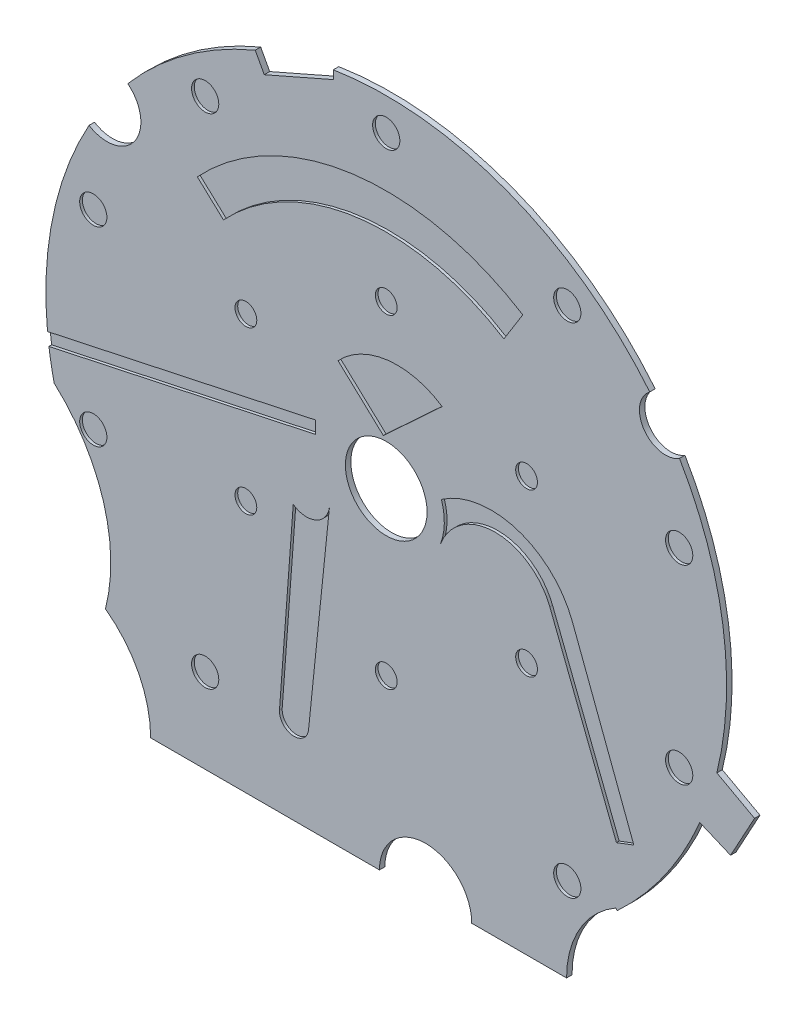
from build123d import *

# Parameters (mm, degrees)
BOSS_EXTRUDE2_DEPTH = 0.2
SKETCH4_R           = 1.5
CUT_EXTRUDE1_DEPTH  = 0.2
SKETCH5_R           = 0.5
CUT_EXTRUDE2_DEPTH  = 0.1
SKETCH6_R           = 0.4
CUT_EXTRUDE3_DEPTH  = 0.1
CUT_EXTRUDE6_DEPTH  = 0.1


with BuildPart() as part:
    # Sketch3 → Boss-Extrude2 (new body)
    with BuildSketch(Plane.XY):
        with BuildLine():
            Line((-8.650876673, -12.25407413), (-0.248745803, -12.25407413))
            ThreePointArc((-0.248745803, -12.25407413), (1.445834978, -10.55949335), (3.140415758, -12.25407413))
            Line((3.140415758, -12.25407413), (6.622856994, -12.25407413))
            ThreePointArc((6.622856994, -12.25407413), (7.105995692, -10.448666248), (8.426264063, -9.125861633))
            Line((8.426264063, -9.125861633), (8.479800816, -9.183843319))
            ThreePointArc((8.479800816, -9.183843319), (10.228299659, -7.185533111), (11.515265421, -4.862989028))
            Line((11.515265421, -4.862989028), (12.645034643, -5.340099639))
            Line((12.645034643, -5.340099639), (13.525538654, -3.725359149))
            Line((13.525538654, -3.725359149), (12.14183381, -2.970836876))
            ThreePointArc((12.14183381, -2.970836876), (12.366623578, 1.821159325), (10.769957457, 6.344920517))
            ThreePointArc((10.769957457, 6.344920517), (9.469693231, 6.602612743), (9.677487695, 7.91177805))
            ThreePointArc((9.677487695, 7.91177805), (4.458067099, 11.67799802), (-1.943326583, 12.348015298))
            Line((-1.943326583, 12.348015298), (-1.943326583, 12.035386554))
            Line((-1.943326583, 12.035386554), (-4.479228025, 10.922703455))
            Line((-4.479228025, 10.922703455), (-4.810432032, 11.537319605))
            ThreePointArc((-4.810432032, 11.537319605), (-7.351587465, 10.109607398), (-9.493012594, 8.132202155))
            ThreePointArc((-9.493012594, 8.132202155), (-9.234137218, 6.438374568), (-10.912999752, 6.095607961))
            ThreePointArc((-10.912999752, 6.095607961), (-12.370451822, 1.794971228), (-12.195428383, -2.742540164))
            ThreePointArc((-12.195428383, -2.742540164), (-10.385309853, -5.600254803), (-10.310731268, -8.98219213))
            ThreePointArc((-10.310731268, -8.98219213), (-9.089572731, -10.419658072), (-8.650876673, -12.25407413))
        make_face()
    extrude(amount=BOSS_EXTRUDE2_DEPTH)

    # Sketch4 → Cut-Extrude1 (cut)
    with BuildSketch(Plane.XY.offset(0.2)):
        Circle(SKETCH4_R)
    extrude(amount=-CUT_EXTRUDE1_DEPTH, mode=Mode.SUBTRACT)

    # Sketch5 → Cut-Extrude2 (cut)
    with BuildSketch(Plane.XY.offset(0.2)):
        with Locations((0, 11.311857504)):
            Circle(SKETCH5_R)
        with Locations((6.648943017, 9.151484959)):
            Circle(SKETCH5_R)
        with Locations((10.75821579, 3.495556207)):
            Circle(SKETCH5_R)
        with Locations((10.75821579, -3.495556207)):
            Circle(SKETCH5_R)
        with Locations((6.648943017, -9.151484959)):
            Circle(SKETCH5_R)
        with Locations((-6.648943017, -9.151484959)):
            Circle(SKETCH5_R)
        with Locations((-10.75821579, -3.495556207)):
            Circle(SKETCH5_R)
        with Locations((-10.75821579, 3.495556207)):
            Circle(SKETCH5_R)
        with Locations((-6.648943017, 9.151484959)):
            Circle(SKETCH5_R)
    extrude(amount=-CUT_EXTRUDE2_DEPTH, mode=Mode.SUBTRACT)

    # Sketch6 → Cut-Extrude3 (cut)
    with BuildSketch(Plane.XY.offset(0.2)):
        with Locations((0, 5.951320454)):
            Circle(SKETCH6_R)
        with Locations((5.153994699, 2.975660227)):
            Circle(SKETCH6_R)
        with Locations((5.153994699, -2.975660227)):
            Circle(SKETCH6_R)
        with Locations((0, -5.951320454)):
            Circle(SKETCH6_R)
        with Locations((-5.153994699, -2.975660227)):
            Circle(SKETCH6_R)
        with Locations((-5.153994699, 2.975660227)):
            Circle(SKETCH6_R)
    extrude(amount=-CUT_EXTRUDE3_DEPTH, mode=Mode.SUBTRACT)

    # Sketch7 → Cut-Extrude6 (cut)
    with BuildSketch(Plane.XY.offset(0.2)):
        with BuildLine():
            Line((-6.937396584, 6.446885446), (-6.51899849, 6.058070341))
            ThreePointArc((-6.51899849, 6.058070341), (-1.17077586, 8.821952247), (4.713219322, 7.548716526))
            Line((4.713219322, 7.548716526), (5.01572008, 8.033203309))
            ThreePointArc((5.01572008, 8.033203309), (-1.245917829, 9.388157012), (-6.937396584, 6.446885446))
        make_face()
        with BuildLine():
            Line((-6.51899849, 6.058070341), (-5.97717014, 5.554552161))
            ThreePointArc((-5.97717014, 5.554552161), (-1.073466502, 8.088713263), (4.321478804, 6.921302879))
            Line((4.321478804, 6.921302879), (4.713219322, 7.548716526))
            ThreePointArc((4.713219322, 7.548716526), (-1.17077586, 8.821952247), (-6.51899849, 6.058070341))
        make_face()
        Polygon((-13.213392068, -1.849616731), (-2.596608573, 0.423918438), (-2.596608573, 0.882797096), (-13.213392068, -1.390738073), align=None)
        with BuildLine():
            Line((-2.850848357, -9.076740417), (-2.081840804, -1.604013127))
            ThreePointArc((-2.081840804, -1.604013127), (-2.574626592, -2.289398349), (-3.41503625, -2.210011057))
            Line((-3.41503625, -2.210011057), (-3.920034525, -8.997187875))
            ThreePointArc((-3.920034525, -8.997187875), (-3.425217712, -9.571557231), (-2.850848357, -9.076740417))
        make_face()
        with BuildLine():
            ThreePointArc((-1.770469413, 3.181469047), (0.058709144, 4.110808601), (2.054752369, 3.636069044))
            Line((2.054752369, 3.636069044), (-0.105672739, 1.633878875))
            Line((-0.105672739, 1.633878875), (-1.770469413, 3.181469047))
        make_face()
        with BuildLine():
            ThreePointArc((1.990756871, -0.766161232), (2.132467077, -0.05196268), (2.025710728, 0.668290355))
            ThreePointArc((2.025710728, 0.668290355), (4.794865348, 1.103096967), (6.836930945, -0.817122344))
            Line((6.836930945, -0.817122344), (9.092520301, -6.792589594))
            Line((9.092520301, -6.792589594), (8.454091655, -7.033580432))
            Line((8.454091655, -7.033580432), (6.007993214, -0.757608342))
            ThreePointArc((6.007993214, -0.757608342), (3.996445347, 0.614174349), (1.990756871, -0.766161232))
        make_face()
    extrude(amount=-CUT_EXTRUDE6_DEPTH, mode=Mode.SUBTRACT)


solid = part.part
